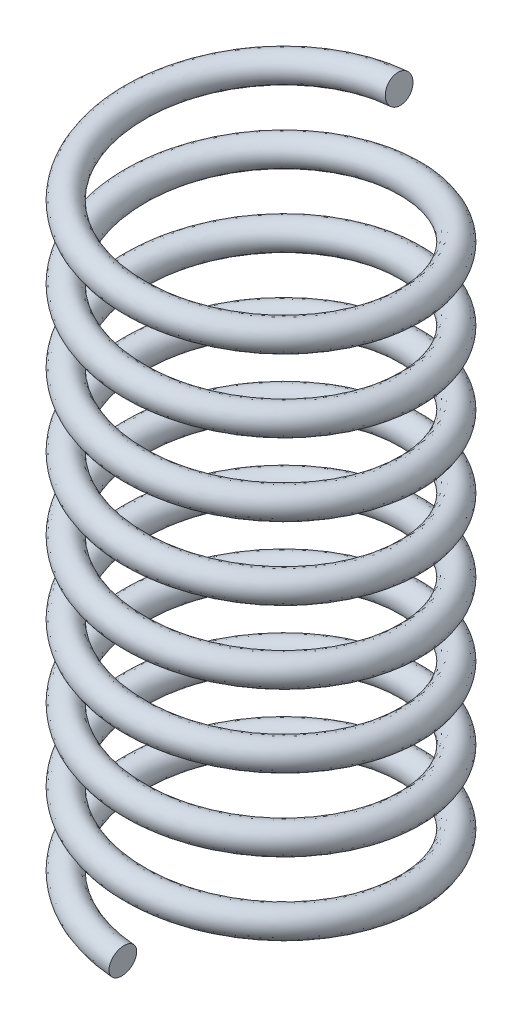
SolidWorks part; units mm, degrees
ref_plane "Front Plane" through (0, 0, 0) normal (0, 0, 1) x (1, 0, 0)
ref_plane "Top Plane" through (0, 0, 0) normal (0, 1, 0) x (1, 0, 0)
ref_plane "Right Plane" through (0, 0, 0) normal (1, 0, 0) x (0, 0, -1)
other "Configuration Table"
sketch "Sketch1" plane through (0, 0, 0) normal (0, 1, 0) x (1, 0, 0)
  line L0 (0, 0) -> (0, 21.7386) construction
  circle A0 centre (0, 0) radius 12.5
  dimension "D1" = 25
curve "Helix/Spiral1" pitch 6.5588 height 55.75 turns 8.5
ref_plane "Plane1" through (0, 0, 12.5) normal (-0.9965, 0.0832, 0) x (0, 0, 1)
sketch "Sketch2" plane through (0, 0, 12.5) normal (-0.9965, 0.0832, 0) x (0, 0, 1)
  circle A0 centre (-0.0172, 0) radius 1.25
  dimension "D1" = 2.5
sweep "Sweep1" add profiles "Sketch2" path "Helix/Spiral1"
sketch "Sketch3" plane through (0, 0, 0) normal (1, 0, 0) x (0, 0, -1)
  line L0 (0, 0) -> (0, 63.6732)
